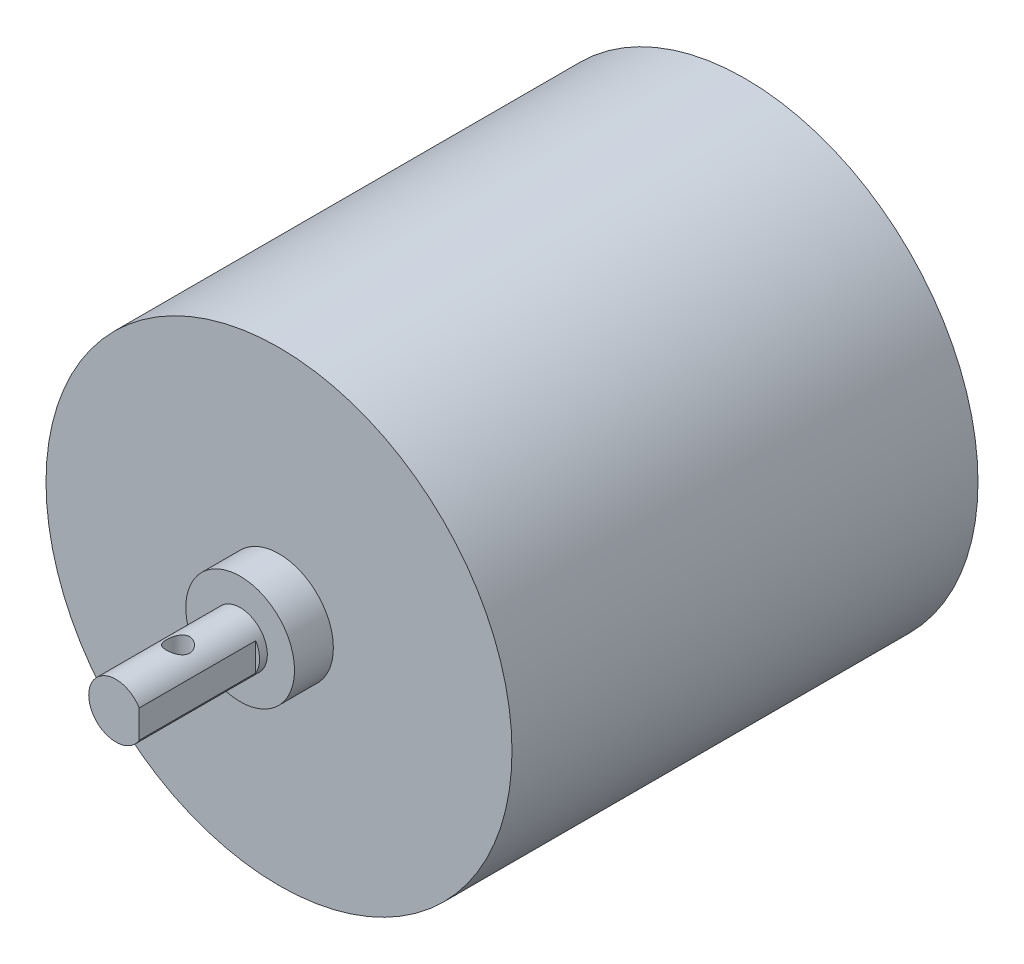
from build123d import *

# Parameters (mm, degrees)
SKETCH_1_R          = 30
EXTRUDE_1_DEPTH     = 60
SKETCH_2_R          = 7
EXTRUDE_2_DEPTH     = 5
SKETCH_3_R          = 3.5
EXTRUDE_3_DEPTH     = 16
CUT_EXTRUDE_START   = -15
CUT_EXTRUDE_1_DEPTH = 15
SKETCH_5_R          = 1.5
CUT_EXTRUDE_2_DEPTH = 7.5


with BuildPart() as part:
    # 草图1 → 凸台-拉伸1 (new body)
    with BuildSketch(Plane.XY):
        Circle(SKETCH_1_R)
    extrude(amount=EXTRUDE_1_DEPTH)

    # 草图2 → 凸台-拉伸2 (add)
    with BuildSketch(Plane.XY.offset(60)):
        Circle(SKETCH_2_R)
    extrude(amount=EXTRUDE_2_DEPTH)

    # 草图3 → 凸台-拉伸3 (add)
    with BuildSketch(Plane.XY.offset(65)):
        Circle(SKETCH_3_R)
    extrude(amount=EXTRUDE_3_DEPTH)

    # 草图4 → 切除-拉伸1 (cut)
    with BuildSketch(Plane.XY.offset(81).offset(CUT_EXTRUDE_START)):
        with BuildLine():
            ThreePointArc((3.5, 0), (3.372684391, 0.935414347), (3, 1.802775638))
            Line((3, 1.802775638), (3, 0))
            Line((3, 0), (3.5, 0))
        make_face()
        with BuildLine():
            Line((3.5, 0), (3, 0))
            Line((3, 0), (3, -1.802775638))
            ThreePointArc((3, -1.802775638), (3.372684391, -0.935414347), (3.5, 0))
        make_face()
    extrude(amount=CUT_EXTRUDE_1_DEPTH, mode=Mode.SUBTRACT)

    # 草图5 → 切除-拉伸2 (cut, symmetric)
    with BuildSketch(Plane(origin=(3, 0, 0), x_dir=(0, 0, -1), z_dir=(0, -1, 0))):
        with Locations((-73, -3)):
            Circle(SKETCH_5_R)
    extrude(amount=CUT_EXTRUDE_2_DEPTH, both=True, mode=Mode.SUBTRACT)


solid = part.part
